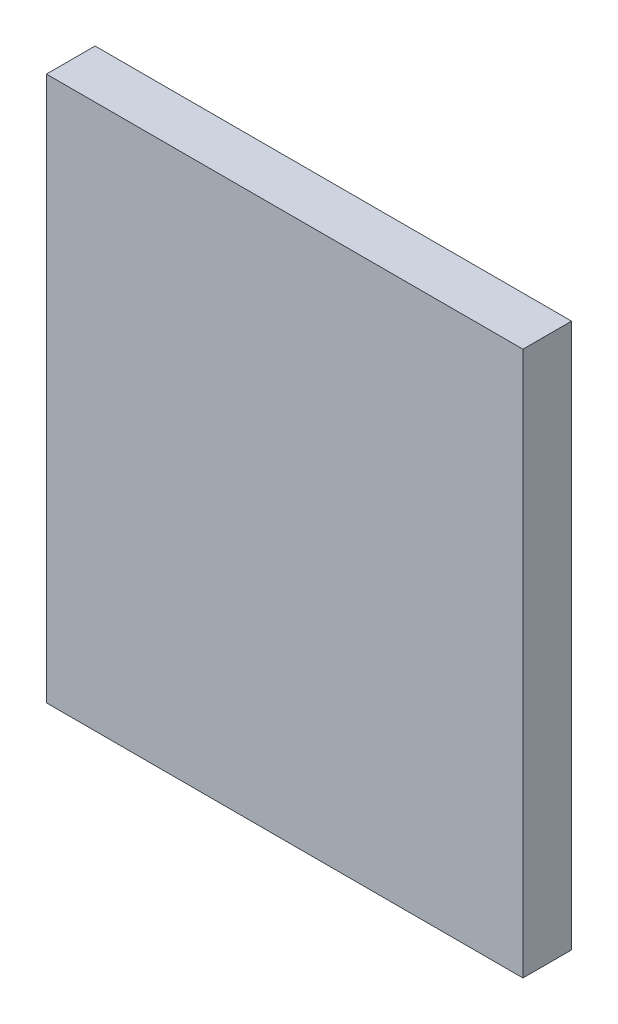
from build123d import *

# Parameters (mm, degrees)
SKETCH_1_W      = 245
SKETCH_1_H      = 280
EXTRUDE_1_DEPTH = 25


with BuildPart() as part:
    # 草图1 → 凸台-拉伸1 (new body)
    with BuildSketch(Plane.XY):
        Rectangle(SKETCH_1_W, SKETCH_1_H)
    extrude(amount=EXTRUDE_1_DEPTH)


solid = part.part
